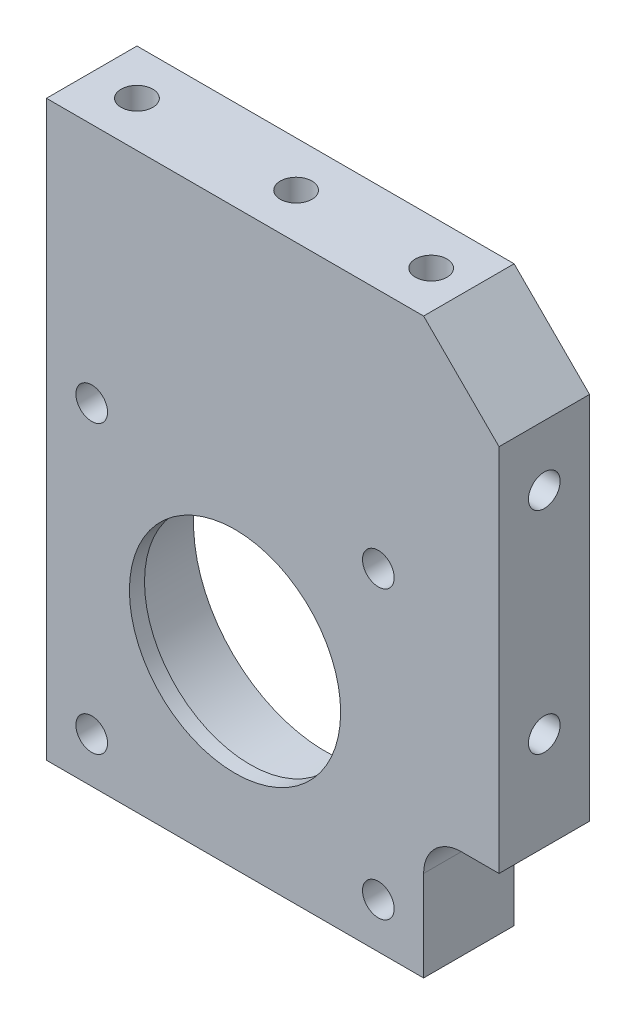
SolidWorks part; units mm, degrees
material "6061Al"
ref_plane "前视基准面" through (0, 0, 0) normal (0, 0, 1) x (1, 0, 0)
ref_plane "上视基准面" through (0, 0, 0) normal (0, 1, 0) x (1, 0, 0)
ref_plane "右视基准面" through (0, 0, 0) normal (1, 0, 0) x (0, 0, -1)
sketch "草图1" plane through (0, 0, 0) normal (0, 0, 1) x (1, 0, 0)
  line L1 (-30, -41) -> (30, -41)
  line L2 (-30, -41) -> (-30, 41)
  line L3 (-30, 41) -> (30, 41)
  line L4 (30, -41) -> (30, 41)
  line L5 (-30, -41) -> (30, 41) construction
  line L6 (-30, 41) -> (30, -41) construction
  point P0 (0, 0)
  dimension "D1" = 60
  dimension "D2" = 82
extrude "凸台-拉伸1" add sketch "草图1" along normal mid plane 12
sketch "草图10" plane through (0, 0, -6) normal (0, 0, 1) x (1, 0, 0)
  line L1 (-30, -41) -> (30, -41) construction
  line L2 (-30, 41) -> (-30, -41) construction
  circle A0 centre (-5, -11) radius 17.5
  dimension "D1" = 35
  dimension "D2" = 30
  dimension "D3" = 25
extrude "切除-拉伸1" cut sketch "草图10" along normal blind 10
sketch "草图12" plane through (0, 0, 4) normal (0, 0, -1) x (-1, 0, 0)
  circle A0 centre (5, -11) radius 14
  dimension "D1" = 28
extrude "切除-拉伸2" cut sketch "草图12" against normal through all
sketch "草图13" plane through (0, 0, 6) normal (0, 0, 1) x (1, 0, 0)
  line L0 (-30, -41) -> (30, -41) construction
  line L1 (20, -41) -> (30, -41)
  line L2 (20, -41) -> (20, -19)
  line L3 (20, -19) -> (30, -19)
  line L4 (30, -41) -> (30, -19)
  line L5 (30, -41) -> (30, 41) construction
  line L6 (-30, 41) -> (-30, -41) construction
  line L7 (30, 41) -> (-30, 41) construction
  dimension "D1" = 50
  dimension "D2" = 60
extrude "切除-拉伸3" cut sketch "草图13" against normal through all
fillet "圆角1" radius 5 1 edges at (20, -19, 0)
hole_wizard "M5 螺纹孔1" positions "草图14" profile "草图15" tap size "M5" standard "ISO"
sketch "草图14" plane through (0, 0, 6) normal (0, 0, 1) x (1, 0, 0)
  line L0 (-5, -11) -> (-5, 8) construction
  line L2 (-5, -11) -> (14, -11) construction
  point P0 (-5, 8)
  point P3 (-24, -11)
  point P6 (14, -11)
  point P9 (-5, -30)
sketch "草图15" plane through (-5, 8, 6) normal (1, 0, 0) x (0, -1, 0)
  line L0 (0, 0) -> (0, 12)
  line L1 (0, 12) -> (2.1, 12)
  line L2 (2.1, 12) -> (2.1, 0)
  line L5 (2.1, 0) -> (0, 0)
  line L11 (0, -6.35) -> (0, 107.95) construction
  dimension "通孔螺纹孔钻头直径" = 4.2
  dimension "通孔螺纹孔钻头深度" = 12
cosmetic thread "孔螺蚊线1" [suppressed] parameters "D2"=5
cosmetic thread "孔螺蚊线2" [suppressed] parameters "D2"=5
cosmetic thread "孔螺蚊线3" [suppressed] parameters "D2"=5
cosmetic thread "孔螺蚊线4" [suppressed] parameters "D2"=5
hole_wizard "M5 螺纹孔2" positions "草图16" profile "草图17" tap size "M5" standard "ISO" end condition through all
sketch "草图16" plane through (0, 0, -6) normal (0, 0, -1) x (-1, 0, 0)
  circle A0 centre (5, -11) radius 14 construction
  point P0 (-14, 8)
  point P3 (-14, -30)
  point P6 (24, -30)
  point P9 (24, 8)
sketch "草图17" plane through (14, 8, -6) normal (1, 0, 0) x (0, 1, 0)
  line L0 (0, 0) -> (0, 12)
  line L1 (0, 12) -> (2.1, 12)
  line L2 (2.1, 12) -> (2.1, 0)
  line L5 (2.1, 0) -> (0, 0)
  line L11 (0, -6.35) -> (0, 107.95) construction
  dimension "通孔螺纹孔钻头直径" = 4.2
  dimension "通孔螺纹孔钻头深度" = 12
cosmetic thread "孔螺蚊线5" parameters "D2"=5
cosmetic thread "孔螺蚊线6" parameters "D2"=5
cosmetic thread "孔螺蚊线7" parameters "D2"=5
cosmetic thread "孔螺蚊线8" parameters "D2"=5
other "移动面1" face at (0, 41, 0) parameters "D1"=1
other "移动面2" [suppressed] parameters "D1"=8
chamfer "倒角2" distance 10 angle 45 1 edges at (30, 40, 0)
hole_wizard "M5 螺纹孔3" positions "草图18" profile "草图19" tap size "M5" standard "ISO"
sketch "草图18" plane through (0, 40, 0) normal (0, 1, 0) x (1, 0, 0)
  line L3 (-30, -6) -> (-30, 6) construction
  line L4 (20, -6) -> (20, 6) construction
  point P12 (-24, 0)
  point P17 (23, 0)
  point P18 (-2.9, 0)
  point P20 (15, 0)
  point P41 (0, 0)
  dimension "D1" = 6
  dimension "D3" = 21.1
  dimension "D2" = 5
sketch "草图19" plane through (-24, 40, 0) normal (1, 0, 0) x (0, 0, 1)
  line L0 (0, 0) -> (0, 13.6618)
  line L1 (0, 13.6618) -> (2.1, 12.4)
  line L2 (2.1, 12.4) -> (2.1, 0)
  line L5 (2.1, 0) -> (0, 0)
  line L10 (0, 13.6618) -> (-2.1, 12.4) construction
  line L11 (0, -6.35) -> (0, 107.95) construction
  dimension "螺纹孔钻头直径" = 4.2
  dimension "螺纹孔钻头深度" = 12.4
  dimension "导头角度" = 118
cosmetic thread "孔螺蚊线9" parameters "D1"=10, "D2"=5
cosmetic thread "孔螺蚊线14" parameters "D1"=10, "D2"=5
cosmetic thread "孔螺蚊线15" parameters "D1"=10, "D2"=5
hole_wizard "M5 螺纹孔4" positions "草图22" profile "草图23" tap size "M5" standard "ISO"
sketch "草图22" plane through (30, 0, 0) normal (1, 0, 0) x (0, 0, -1)
  line L0 (0, 30) -> (0, -19) construction
  line L1 (6, 30) -> (-6, 30) construction
  line L2 (6, -19) -> (-6, -19) construction
  line L4 (-6, 40) -> (6, 40) construction
  point P0 (0, 22)
  point P2 (0, -6)
  dimension "D1" = 18
  dimension "D2" = 28
sketch "草图23" plane through (30, 22, 0) normal (0, 1, 0) x (0, 0, -1)
  line L0 (0, 0) -> (0, 13.6618)
  line L1 (0, 13.6618) -> (2.1, 12.4)
  line L2 (2.1, 12.4) -> (2.1, 0)
  line L5 (2.1, 0) -> (0, 0)
  line L10 (0, 13.6618) -> (-2.1, 12.4) construction
  line L11 (0, -6.35) -> (0, 107.95) construction
  dimension "螺纹孔钻头直径" = 4.2
  dimension "螺纹孔钻头深度" = 12.4
  dimension "导头角度" = 118
cosmetic thread "孔螺蚊线12" parameters "D1"=10, "D2"=5
cosmetic thread "孔螺蚊线13" parameters "D1"=10, "D2"=5
other "移动面3" face at (-5, -41, 0) parameters "D1"=5
equation "\"D2@草图14\"=\"D1@草图14\""
equation "\"D1@草图16\"=\"D2@草图16\""
